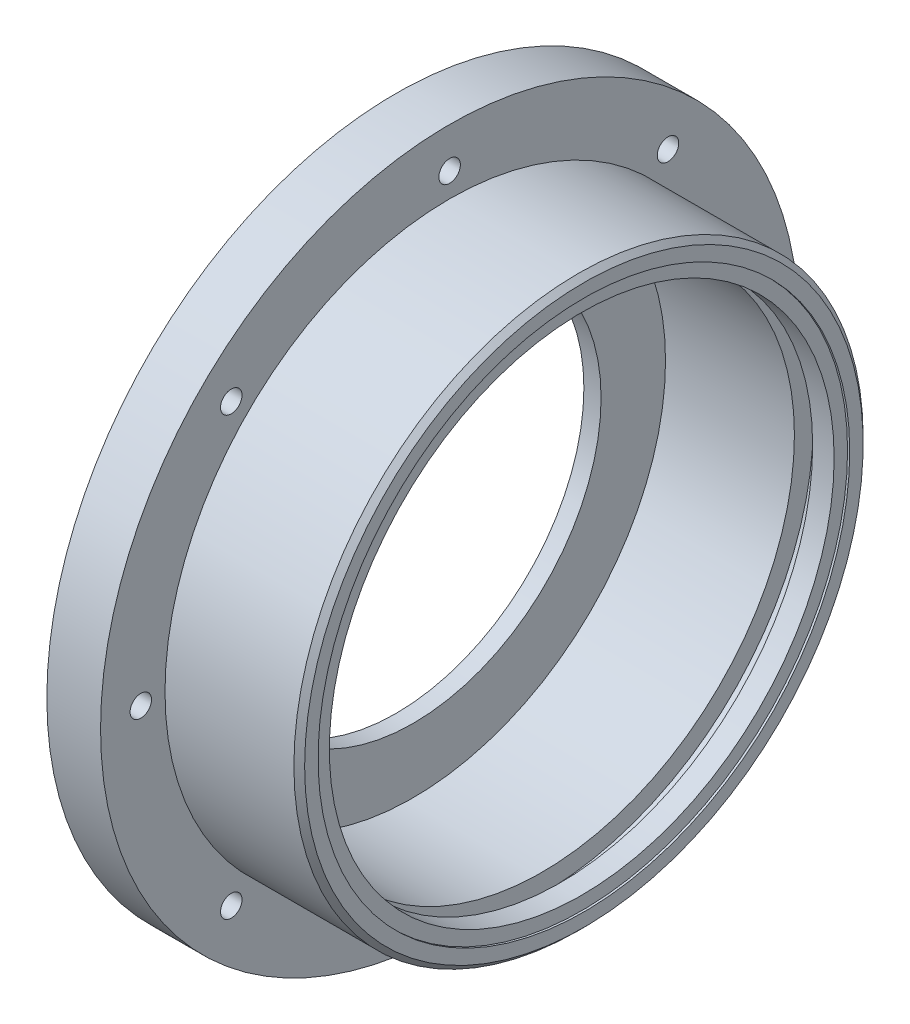
from build123d import *

# Parameters (mm, degrees)
SKETCH_2_W          = 20
SKETCH_2_H          = 65
SKETCH_3_W          = 25
SKETCH_3_H          = 53
SKETCH_6_R          = 35
CUT_EXTRUDE_1_DEPTH = 103.347447452
CUT_EXTRUDE_START   = 13.2
SKETCH_7_R          = 47
CUT_EXTRUDE_2_DEPTH = 90.147447452
CUT_EXTRUDE_START_2 = 40.6
SKETCH_10_R         = 50.5
CUT_EXTRUDE_4_DEPTH = 3.4
SKETCH_15_R         = 65
CUT_EXTRUDE_6_DEPTH = 10
CUT_EXTRUDE_START_3 = 44.6
SKETCH_12_R         = 49.5
CUT_EXTRUDE_5_DEPTH = 58.747447452
SKETCH_16_R         = 2
CUT_EXTRUDE_7_DEPTH = 99.361577865
CHAMFER_1_SIZE      = 1


with BuildPart() as part:
    # 草图2 → 旋转-薄壁1 (revolve)
    with BuildSketch(Plane.XY, mode=Mode.PRIVATE) as revolve_1_sk:
        with Locations((10, 32.5)):
            Rectangle(SKETCH_2_W, SKETCH_2_H)
    revolve(revolve_1_sk.sketch.rotate(Axis((0, 0, 0), (1, 0, 0)), 90), axis=Axis((0, 0, 0), (1, 0, 0)))

    # 草图3 → 旋转-薄壁2 (revolve)
    with BuildSketch(Plane.XY, mode=Mode.PRIVATE) as revolve_2_sk:
        with Locations((32.5, 26.5)):
            Rectangle(SKETCH_3_W, SKETCH_3_H)
    revolve(revolve_2_sk.sketch.rotate(Axis((20, 0, 0), (1, 0, 0)), 90), axis=Axis((20, 0, 0), (1, 0, 0)))

    # 草图6 → 切除-拉伸1 (cut, through all)
    with BuildSketch(Plane(origin=(0, 0, 0), x_dir=(0, 0, -1), z_dir=(1, 0, 0))):
        with Locations(Location((0, 0, 0), (0, 0, 180))):
            Circle(SKETCH_6_R)
    extrude(amount=CUT_EXTRUDE_1_DEPTH, mode=Mode.SUBTRACT)

    # 草图7 → 切除-拉伸2 (cut, through all)
    with BuildSketch(Plane(origin=(0, 0, 0), x_dir=(0, 0, -1), z_dir=(1, 0, 0)).offset(CUT_EXTRUDE_START)):
        Circle(SKETCH_7_R)
    extrude(amount=CUT_EXTRUDE_2_DEPTH, mode=Mode.SUBTRACT)

    # 草图10 → 切除-拉伸4 (cut)
    with BuildSketch(Plane(origin=(0, 0, 0), x_dir=(0, 0, -1), z_dir=(1, 0, 0)).offset(CUT_EXTRUDE_START_2)):
        Circle(SKETCH_10_R)
    extrude(amount=-CUT_EXTRUDE_4_DEPTH, mode=Mode.SUBTRACT)

    # 草图15 → 切除-拉伸6 (cut)
    with BuildSketch(Plane(origin=(0, 0, 0), x_dir=(0, 0, -1), z_dir=(1, 0, 0))):
        with Locations(Location((0, 0, 0), (0, 0, 180))):
            Circle(SKETCH_15_R)
    extrude(amount=CUT_EXTRUDE_6_DEPTH, mode=Mode.SUBTRACT)

    # 草图12 → 切除-拉伸5 (cut, through all)
    with BuildSketch(Plane(origin=(0, 0, 0), x_dir=(0, 0, -1), z_dir=(1, 0, 0)).offset(CUT_EXTRUDE_START_3)):
        Circle(SKETCH_12_R)
    extrude(amount=CUT_EXTRUDE_5_DEPTH, mode=Mode.SUBTRACT)

    # 草图16 → 切除-拉伸7 (cut, through all)
    with BuildSketch(Plane.ZY.offset(-10)):
        with Locations((0, 57.5)):
            Circle(SKETCH_16_R)
        with Locations((40.658639918, 40.658639918)):
            Circle(SKETCH_16_R)
        with Locations((57.5, 0)):
            Circle(SKETCH_16_R)
        with Locations((40.658639918, -40.658639918)):
            Circle(SKETCH_16_R)
        with Locations((0, -57.5)):
            Circle(SKETCH_16_R)
        with Locations((-40.658639918, -40.658639918)):
            Circle(SKETCH_16_R)
        with Locations((-57.5, 0)):
            Circle(SKETCH_16_R)
        with Locations((-40.658639918, 40.658639918)):
            Circle(SKETCH_16_R)
    extrude(amount=-CUT_EXTRUDE_7_DEPTH, mode=Mode.SUBTRACT)

    # 倒角1
    chamfer_1_edges = [part.edges().sort_by_distance(p)[0] for p in [
        (45, 0, -53),
    ]]
    chamfer(chamfer_1_edges, length=CHAMFER_1_SIZE)


solid = part.part
